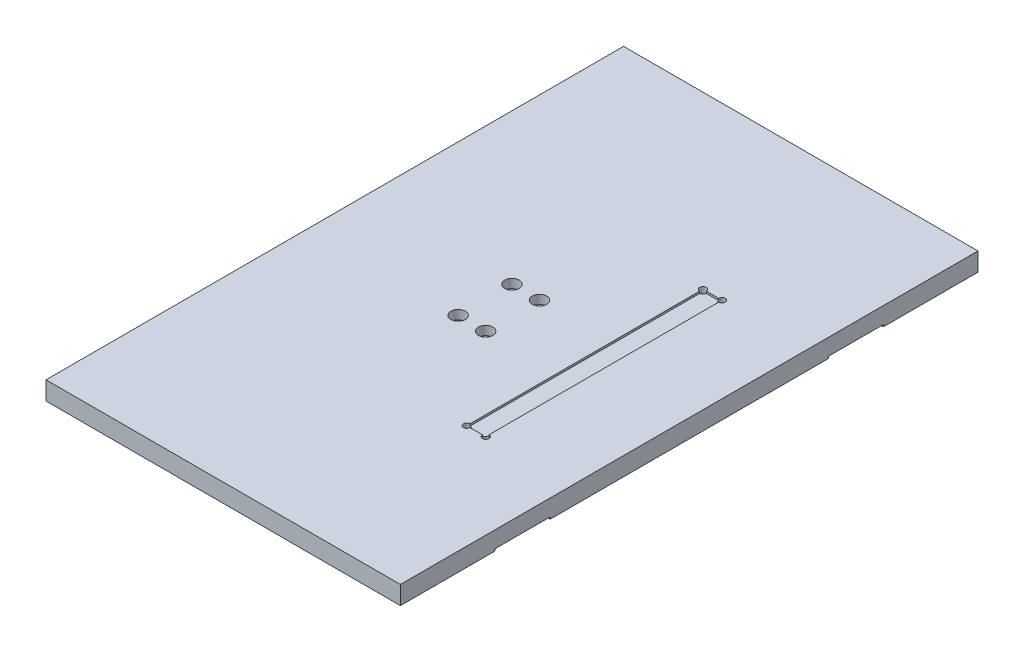
from build123d import *

# Parameters (mm, degrees)
SKETCH_1_W                = 270
SKETCH_1_H                = 440
EXTRUDE_1_DEPTH           = 14
SKETCH_2_W                = 270
SKETCH_2_H                = 42
CUT_EXTRUDE_1_DEPTH       = 1.5
HOLE_WIZARD_1_D           = 6.6
HOLE_WIZARD_1_CBORE_D     = 11
HOLE_WIZARD_1_CBORE_DEPTH = 6.8
SKETCH_4_W                = 14.5
SKETCH_4_H                = 180
CUT_EXTRUDE_2_DEPTH       = 1.5
CUT_EXTRUDE_3_REACH       = 260.498
SKETCH_5_R                = 2.5


with BuildPart() as part:
    # 草图1 → 凸台-拉伸1 (new body)
    with BuildSketch(Plane(origin=(0, 0, 0), x_dir=(1, 0, 0), z_dir=(0, 1, 0))):
        Rectangle(SKETCH_1_W, SKETCH_1_H)
    extrude(amount=EXTRUDE_1_DEPTH)

    # 草图2 → 切除-拉伸1 (cut)
    with BuildSketch(Plane.XZ):
        with Locations((0, 127)):
            Rectangle(SKETCH_2_W, SKETCH_2_H)
        with Locations((0, -127)):
            Rectangle(SKETCH_2_W, SKETCH_2_H)
    extrude(amount=-CUT_EXTRUDE_1_DEPTH, mode=Mode.SUBTRACT)

    # 打孔尺寸(%根据)内六角圆柱头螺钉的类型1 (through all)
    with Locations(Plane(origin=(-20.55, 14, 20.5), x_dir=(0, 0, 1), z_dir=(0, 1, 0))):
        with Locations((0, 0), (-41, 0), (0, 21), (-41, 21)):
            CounterBoreHole(HOLE_WIZARD_1_D / 2, HOLE_WIZARD_1_CBORE_D / 2, HOLE_WIZARD_1_CBORE_DEPTH)

    # 草图4 → 切除-拉伸2 (cut)
    with BuildSketch(Plane(origin=(0, 14, 0), x_dir=(1, 0, 0), z_dir=(0, 1, 0))):
        with Locations((62.75, 0)):
            Rectangle(SKETCH_4_W, SKETCH_4_H)
    extrude(amount=-CUT_EXTRUDE_2_DEPTH, mode=Mode.SUBTRACT)

    # 草图5 → 切除-拉伸3 (cut, up to next)
    with BuildSketch(Plane(origin=(0, 14, 0), x_dir=(1, 0, 0), z_dir=(0, 1, 0)), mode=Mode.PRIVATE) as cut_extrude_3_sk1:
        with Locations(Location((55.5, 90, 0), (0, 0, 270))):
            Circle(SKETCH_5_R)
    cut_extrude_3_tool1 = extrude(cut_extrude_3_sk1.sketch, amount=-CUT_EXTRUDE_3_REACH, mode=Mode.PRIVATE) & part.part
    # 草图5 → 切除-拉伸3 (cut, up to next)
    with BuildSketch(Plane(origin=(0, 14, 0), x_dir=(1, 0, 0), z_dir=(0, 1, 0)), mode=Mode.PRIVATE) as cut_extrude_3_sk2:
        with Locations(Location((70, 90, 0), (0, 0, 270))):
            Circle(SKETCH_5_R)
    cut_extrude_3_tool2 = extrude(cut_extrude_3_sk2.sketch, amount=-CUT_EXTRUDE_3_REACH, mode=Mode.PRIVATE) & part.part
    # 草图5 → 切除-拉伸3 (cut, up to next)
    with BuildSketch(Plane(origin=(0, 14, 0), x_dir=(1, 0, 0), z_dir=(0, 1, 0)), mode=Mode.PRIVATE) as cut_extrude_3_sk3:
        with Locations(Location((55.5, -90, 0), (0, 0, 90))):
            Circle(SKETCH_5_R)
    cut_extrude_3_tool3 = extrude(cut_extrude_3_sk3.sketch, amount=-CUT_EXTRUDE_3_REACH, mode=Mode.PRIVATE) & part.part
    # 草图5 → 切除-拉伸3 (cut, up to next)
    with BuildSketch(Plane(origin=(0, 14, 0), x_dir=(1, 0, 0), z_dir=(0, 1, 0)), mode=Mode.PRIVATE) as cut_extrude_3_sk4:
        with Locations(Location((70, -90, 0), (0, 0, 90))):
            Circle(SKETCH_5_R)
    cut_extrude_3_tool4 = extrude(cut_extrude_3_sk4.sketch, amount=-CUT_EXTRUDE_3_REACH, mode=Mode.PRIVATE) & part.part
    add(cut_extrude_3_tool1.solids().sort_by_distance((55.5, 14, -90))[0], mode=Mode.SUBTRACT)
    add(cut_extrude_3_tool2.solids().sort_by_distance((70, 14, -90))[0], mode=Mode.SUBTRACT)
    add(cut_extrude_3_tool3.solids().sort_by_distance((55.5, 14, 90))[0], mode=Mode.SUBTRACT)
    add(cut_extrude_3_tool4.solids().sort_by_distance((70, 14, 90))[0], mode=Mode.SUBTRACT)


solid = part.part
